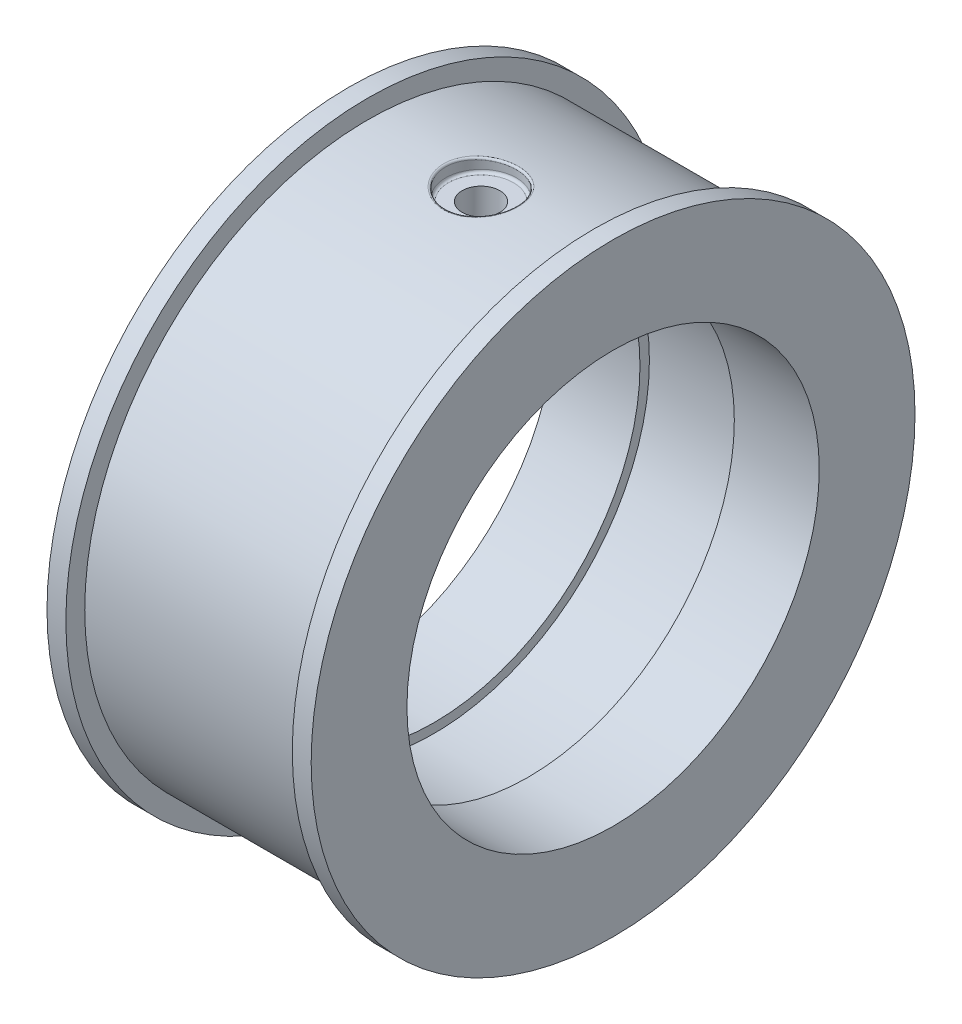
from build123d import *

# Parameters (mm, degrees)
HOLE1_D           = 7.5
HOLE1_DEPTH       = 1.5
HOLE2_REACH       = 73.196
HOLE2_BORE_R      = 2
DOWEL_HOLE1_D     = 4
DOWEL_HOLE1_DEPTH = 4
DOWEL_HOLE1_TIP   = 1.201721238
FILLET1_R         = 0.2
FILLET2_R         = 0.3


with BuildPart() as part:
    # Sketch1 → Revolve1 (revolve)
    with BuildSketch(Plane.XY, mode=Mode.PRIVATE) as revolve1_sk:
        Polygon((-8.389660143, 21.85), (-8.389660143, 32), (-6.389660143, 32), (-6.389660143, 30), (17.610339857, 30), (17.610339857, 32), (19.610339857, 32), (19.610339857, 21.85), (10.610339857, 21.85), (10.610339857, 22.85), (0.610339857, 22.85), (0.610339857, 21.85), align=None)
    revolve(revolve1_sk.sketch.rotate(Axis((-19.036826505, 0, 0), (1, 0, 0)), 90), axis=Axis((-19.036826505, 0, 0), (1, 0, 0)))

    # Hole1
    with Locations(Plane(origin=(0, 30, 0), x_dir=(1, 0, 0), z_dir=(0, 1, 0))):
        with Locations((5.610339857, 0)):
            Hole(HOLE1_D / 2, depth=HOLE1_DEPTH)

    # Hole2 bore → Hole2 (cut, up to next)
    with BuildSketch(Plane(origin=(0, 28.5, 0), x_dir=(1, 0, 0), z_dir=(0, 1, 0)), mode=Mode.PRIVATE) as hole2_sk1:
        with Locations((5.610339857, 0)):
            Circle(HOLE2_BORE_R)
    hole2_tool1 = extrude(hole2_sk1.sketch, amount=-HOLE2_REACH, mode=Mode.PRIVATE) & part.part
    add(hole2_tool1.solids().sort_by_distance((5.61034, 28.5, 0))[0], mode=Mode.SUBTRACT)

    # Dowel Hole1
    with Locations(Plane(origin=(0, -30, 0), x_dir=(-1, 0, 0), z_dir=(0, -1, 0))):
        with Locations((-5.610339857, 0)):
            Hole(DOWEL_HOLE1_D / 2, depth=DOWEL_HOLE1_DEPTH)
            with Locations((0, 0, -(DOWEL_HOLE1_DEPTH + DOWEL_HOLE1_TIP / 2))):  # 118° drill point
                Cone(0, DOWEL_HOLE1_D / 2, DOWEL_HOLE1_TIP, mode=Mode.SUBTRACT)

    # Fillet1
    fillet1_edges = [part.edges().sort_by_distance(p)[0] for p in [
        (9.360339864, 29.999999997, -1e-09),
    ]]
    fillet(fillet1_edges, radius=FILLET1_R)

    # Fillet2
    fillet2_edges = [part.edges().sort_by_distance(p)[0] for p in [
        (9.360339857, 28.5, 0),
    ]]
    fillet(fillet2_edges, radius=FILLET2_R)


solid = part.part
